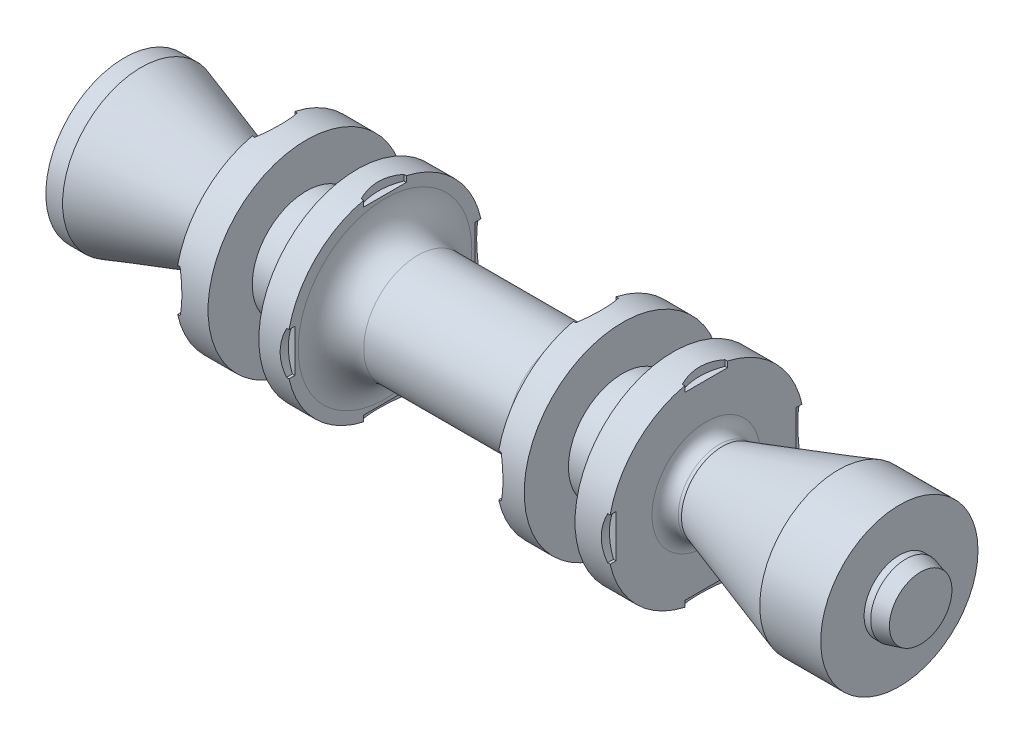
from build123d import *
from OCP.BRepFilletAPI import BRepFilletAPI_MakeChamfer

# Parameters (mm, degrees)
FILLET1_R            = 0.8
FILLET3_R            = 2
CHAMFER1_SIZE        = 0.9
CHAMFER1_SIZE2       = 0.241154273
CUT_EXTRUDE1_START   = 15.5
CUT_EXTRUDE1_DEPTH   = 10
CIRPATTERN1_COUNT    = 4
MIRROR1_START        = 15.5
MIRROR1_COPY_1_DEPTH = 10
MIRROR1_COPY_2_DEPTH = 10
MIRROR1_COPY_3_DEPTH = 10


with BuildPart() as part:
    # Sketch1 → Revolve1 (revolve)
    with BuildSketch(Plane.XY, mode=Mode.PRIVATE) as revolve1_sk:
        Polygon((0, 0), (0, 2.15), (-1.3, 2.15), (-1.3, 4.8), (-5.021327864, 4.8), (-12.1, 2.5), (-13.1, 2.5), (-13.1, 6), (-15.1, 6), (-15.1, 3.3), (-18.2, 3.3), (-18.2, 6), (-19.9, 6), (-19.9, 3.3), (-32.7, 3.3), (-32.7, 6), (-34.4, 6), (-34.4, 3.3), (-37.5, 3.3), (-37.5, 6), (-39.5, 6), (-39.5, 2.5), (-40.5, 2.5), (-47.578672136, 4.8), (-48.6, 4.8), (-48.6, 2.2), (-49.9, 2.2), (-49.9, 0), align=None)
    revolve(revolve1_sk.sketch.rotate(Axis((0, 0, 0), (-1, 0, 0)), 90), axis=Axis((0, 0, 0), (-1, 0, 0)))

    # Fillet1
    fillet1_edges = [part.edges().sort_by_distance(p)[0] for p in [
        (-39.5, 0, 2.5),
        (-13.1, 0, 2.5),
    ]]
    fillet(fillet1_edges, radius=FILLET1_R)

    # Fillet3
    fillet3_edges = [part.edges().sort_by_distance(p)[0] for p in [
        (-32.7, 0, 3.3),
        (-19.9, 0, 3.3),
    ]]
    fillet(fillet3_edges, radius=FILLET3_R)

    # Chamfer1: one chamfer whose edges measure the first distance from different faces: ONE call of the kernel's chamfer builder (chamfer() names one face for all edges)
    chamfer1_edges_1 = [part.edges().sort_by_distance(p)[0] for p in [
        (-49.9, 0, 2.2),
    ]]
    chamfer1_side_1 = [part.faces().sort_by_distance(p)[0] for p in [
        (-49.25, 0, 2.2),
    ]]
    chamfer1_edges_2 = [part.edges().sort_by_distance(p)[0] for p in [
        (0, 0, 2.15),
    ]]
    chamfer1_side_2 = [part.faces().sort_by_distance(p)[0] for p in [
        (-0.65, 0, 2.15),
    ]]
    chamfer1 = BRepFilletAPI_MakeChamfer(part.part.solid().wrapped)
    for e in chamfer1_edges_1:
        chamfer1.Add(CHAMFER1_SIZE, CHAMFER1_SIZE2, e.wrapped, chamfer1_side_1[0].wrapped)  # the first distance lies on this face
    for e in chamfer1_edges_2:
        chamfer1.Add(CHAMFER1_SIZE, CHAMFER1_SIZE2, e.wrapped, chamfer1_side_2[0].wrapped)  # the first distance lies on this face
    add(Compound.cast(chamfer1.Shape()), mode=Mode.REPLACE)

    # Sketch2 → Cut-Extrude1 (cut)
    with BuildSketch(Plane(origin=(0, 0, 0), x_dir=(1, 0, 0), z_dir=(0, 1, 0)).offset(CUT_EXTRUDE1_START)):
        with BuildLine():
            Line((-39.5, 1.3), (-39.35, 1.3))
            ThreePointArc((-39.35, 1.3), (-39.1, 0), (-39.35, -1.3))
            Line((-39.35, -1.3), (-39.5, -1.3))
            Line((-39.5, -1.3), (-39.5, 1.3))
        make_face()
        with BuildLine():
            Line((-32.7, 1.3), (-32.85, 1.3))
            ThreePointArc((-32.85, 1.3), (-33.1, 0), (-32.85, -1.3))
            Line((-32.85, -1.3), (-32.7, -1.3))
            Line((-32.7, -1.3), (-32.7, 1.3))
        make_face()
    cut_extrude1 = extrude(amount=-CUT_EXTRUDE1_DEPTH, mode=Mode.SUBTRACT)

    # CirPattern1: Cut-Extrude1 ×4 about axis
    cirpattern1_axis = Axis((0, 0, 0), (1, 0, 0))
    for i in range(1, CIRPATTERN1_COUNT):
        add(cut_extrude1.rotate(cirpattern1_axis, i * 360 / CIRPATTERN1_COUNT), mode=Mode.SUBTRACT)

    # Mirror1: Cut-Extrude1 across plane
    add(cut_extrude1.mirror(Plane(origin=(-26.3, 0, 0), x_dir=(0, 0, 1), z_dir=(1, 0, 0))), mode=Mode.SUBTRACT)

    # Mirror1 copy 1 sketch → Mirror1 copy 1 (cut)
    with BuildSketch(Plane(origin=(-52.6, 0, 0), x_dir=(-1, 0, 0), z_dir=(0, 0, 1)).offset(MIRROR1_START)):
        with BuildLine():
            Line((-39.5, -1.3), (-39.35, -1.3))
            ThreePointArc((-39.35, -1.3), (-39.1, 0), (-39.35, 1.3))
            Line((-39.35, 1.3), (-39.5, 1.3))
            Line((-39.5, 1.3), (-39.5, -1.3))
        make_face()
        with BuildLine():
            Line((-32.7, -1.3), (-32.85, -1.3))
            ThreePointArc((-32.85, -1.3), (-33.1, 0), (-32.85, 1.3))
            Line((-32.85, 1.3), (-32.7, 1.3))
            Line((-32.7, 1.3), (-32.7, -1.3))
        make_face()
    extrude(amount=-MIRROR1_COPY_1_DEPTH, mode=Mode.SUBTRACT)

    # Mirror1 copy 2 sketch → Mirror1 copy 2 (cut)
    with BuildSketch(Plane(origin=(-52.6, 0, 0), x_dir=(-1, 0, 0), z_dir=(0, -1, 0)).offset(MIRROR1_START)):
        with BuildLine():
            Line((-39.5, -1.3), (-39.35, -1.3))
            ThreePointArc((-39.35, -1.3), (-39.1, 0), (-39.35, 1.3))
            Line((-39.35, 1.3), (-39.5, 1.3))
            Line((-39.5, 1.3), (-39.5, -1.3))
        make_face()
        with BuildLine():
            Line((-32.7, -1.3), (-32.85, -1.3))
            ThreePointArc((-32.85, -1.3), (-33.1, 0), (-32.85, 1.3))
            Line((-32.85, 1.3), (-32.7, 1.3))
            Line((-32.7, 1.3), (-32.7, -1.3))
        make_face()
    extrude(amount=-MIRROR1_COPY_2_DEPTH, mode=Mode.SUBTRACT)

    # Mirror1 copy 3 sketch → Mirror1 copy 3 (cut)
    with BuildSketch(Plane(origin=(-52.6, 0, 0), x_dir=(-1, 0, 0), z_dir=(0, 0, -1)).offset(MIRROR1_START)):
        with BuildLine():
            Line((-39.5, -1.3), (-39.35, -1.3))
            ThreePointArc((-39.35, -1.3), (-39.1, 0), (-39.35, 1.3))
            Line((-39.35, 1.3), (-39.5, 1.3))
            Line((-39.5, 1.3), (-39.5, -1.3))
        make_face()
        with BuildLine():
            Line((-32.7, -1.3), (-32.85, -1.3))
            ThreePointArc((-32.85, -1.3), (-33.1, 0), (-32.85, 1.3))
            Line((-32.85, 1.3), (-32.7, 1.3))
            Line((-32.7, 1.3), (-32.7, -1.3))
        make_face()
    extrude(amount=-MIRROR1_COPY_3_DEPTH, mode=Mode.SUBTRACT)


solid = part.part
